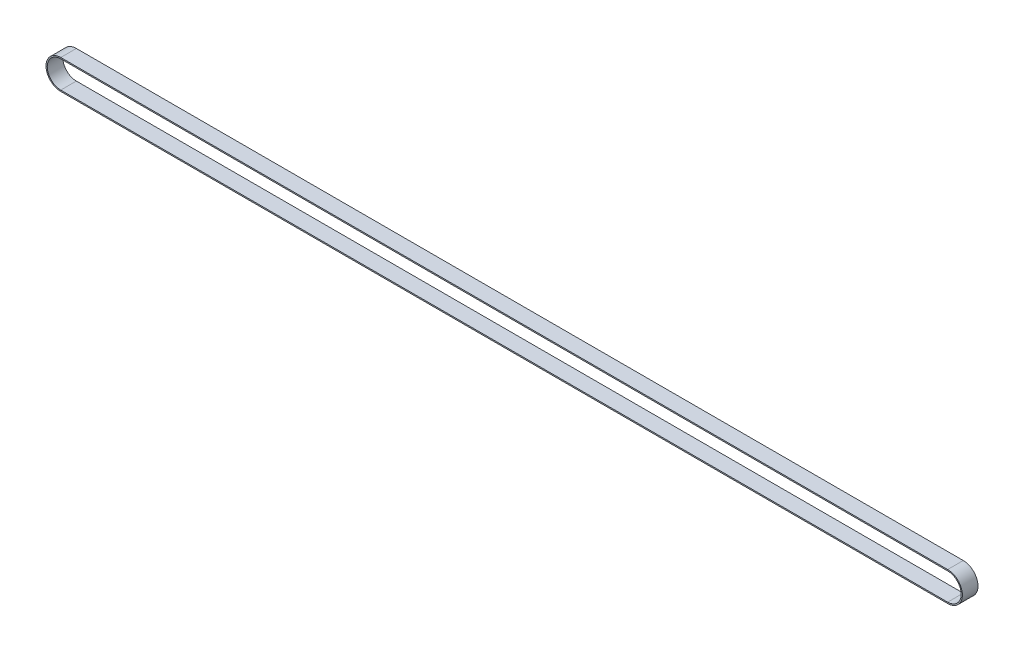
SolidWorks part; units mm, degrees
material "6061 合金"
ref_plane "前视基准面" through (0, 0, 0) normal (0, 0, 1) x (1, 0, 0)
ref_plane "上视基准面" through (0, 0, 0) normal (0, 1, 0) x (1, 0, 0)
ref_plane "右视基准面" through (0, 0, 0) normal (1, 0, 0) x (0, 0, -1)
sketch "草图1" plane through (0, 0, 0) normal (0, 0, 1) x (1, 0, 0)
  line L0 (0, 12.99) -> (852.5, 12.99)
  line L1 (852.5, -12.99) -> (0, -12.99)
  line L2 (0, 14.17) -> (852.5, 14.17)
  line L3 (852.5, -14.17) -> (0, -14.17)
  arc A0 (0, 12.99) -> (0, -12.99) centre (0, 0) ccw
  arc A1 (852.5, -12.99) -> (852.5, 12.99) centre (852.5, 0) ccw
  arc A2 (852.5, -14.17) -> (852.5, 14.17) centre (852.5, 0) ccw
  arc A3 (0, 14.17) -> (0, -14.17) centre (0, 0) ccw
  dimension "D1" = 25.98
  dimension "D2" = 25.98
  dimension "D3" = 852.5
  dimension "D4" = 1.18
extrude "凸台-拉伸1" add sketch "草图1" along normal mid plane 15
